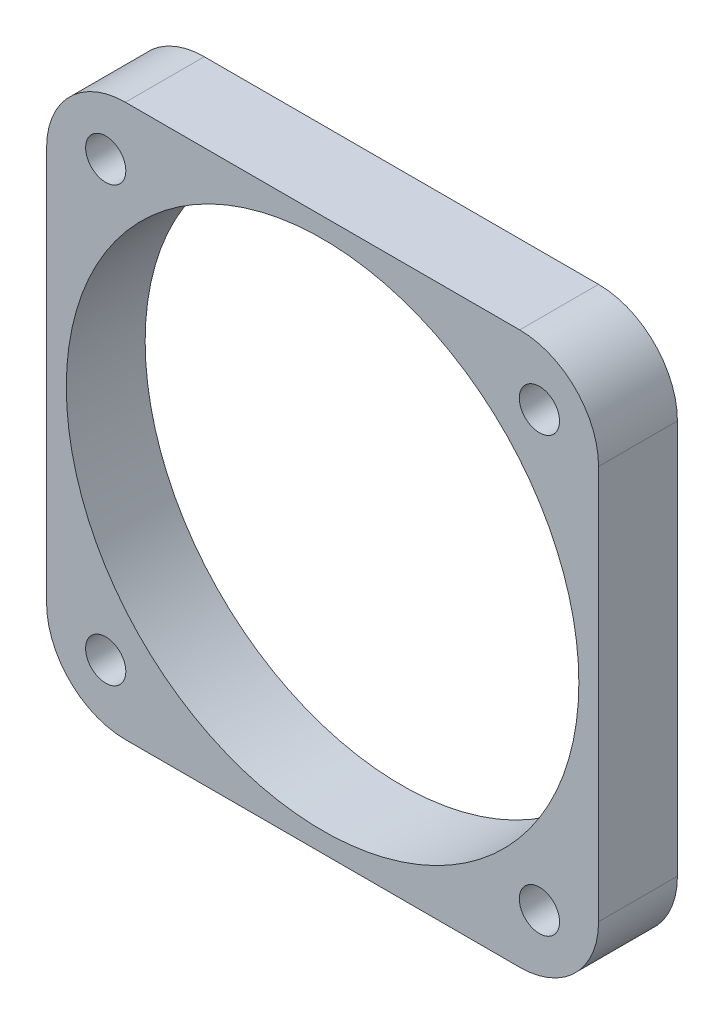
from build123d import *

# Parameters (mm, degrees)
SKETCH1_R              = 65
BOSS_EXTRUDE1_DEPTH    = 20
M12_TAPPED_HOLE1_D     = 10.2
M12_TAPPED_HOLE1_DEPTH = 16
M12_TAPPED_HOLE1_TIP   = 3.064389157


with BuildPart() as part:
    # Sketch1 → Boss-Extrude1 (new body)
    with BuildSketch(Plane.XY):
        with BuildLine():
            Line((20, 0), (120, 0))
            ThreePointArc((120, 0), (134.142135624, 5.857864376), (140, 20))
            Line((140, 20), (140, 120))
            ThreePointArc((140, 120), (134.142135624, 134.142135624), (120, 140))
            Line((120, 140), (20, 140))
            ThreePointArc((20, 140), (5.857864376, 134.142135624), (0, 120))
            Line((0, 120), (0, 20))
            ThreePointArc((0, 20), (5.857864376, 5.857864376), (20, 0))
        make_face()
        with Locations((70, 70)):
            Circle(SKETCH1_R, mode=Mode.SUBTRACT)
    extrude(amount=BOSS_EXTRUDE1_DEPTH)

    # M12 Tapped Hole1
    with Locations(Plane(origin=(15, 125, 20), x_dir=(1, 0, 0), z_dir=(0, 0, 1))):
        with Locations((0, 0), (110, 0), (110, -110), (0, -110)):
            Hole(M12_TAPPED_HOLE1_D / 2, depth=M12_TAPPED_HOLE1_DEPTH)
            with Locations((0, 0, -(M12_TAPPED_HOLE1_DEPTH + M12_TAPPED_HOLE1_TIP / 2))):  # 118° drill point
                Cone(0, M12_TAPPED_HOLE1_D / 2, M12_TAPPED_HOLE1_TIP, mode=Mode.SUBTRACT)


solid = part.part
